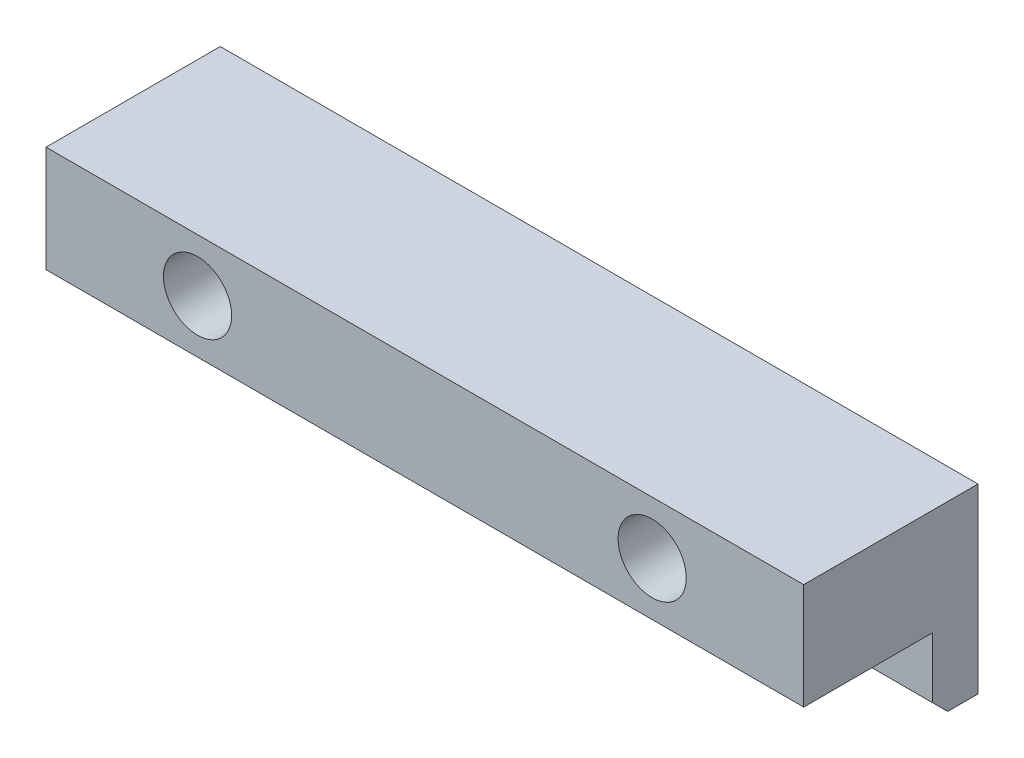
from build123d import *

# Parameters (mm, degrees)
SKETCH1_W           = 50
SKETCH1_H           = 12
BOSS_EXTRUDE1_DEPTH = 5
SKETCH2_R           = 2.25
CUT_EXTRUDE1_DEPTH  = 52.662365412
SKETCH3_W           = 2
SKETCH3_H           = 5
CUT_EXTRUDE2_DEPTH  = 52.662365412
CHAMFER1_SIZE       = 1
MOVE_FACE1_BY       = 6.5


with BuildPart() as part:
    # Sketch1 → Boss-Extrude1 (new body)
    with BuildSketch(Plane.XY):
        with Locations((25, 6)):
            Rectangle(SKETCH1_W, SKETCH1_H)
    extrude(amount=BOSS_EXTRUDE1_DEPTH)

    # Sketch2 → Cut-Extrude1 (cut, through all)
    with BuildSketch(Plane.XY.offset(5)):
        with Locations((10, 8.5)):
            Circle(SKETCH2_R)
        with Locations((40, 8.5)):
            Circle(SKETCH2_R)
    extrude(amount=-CUT_EXTRUDE1_DEPTH, mode=Mode.SUBTRACT)

    # Sketch3 → Cut-Extrude2 (cut, through all)
    with BuildSketch(Plane(origin=(50, 0, 0), x_dir=(0, 0, -1), z_dir=(1, 0, 0))):
        with Locations((-4, 2.5)):
            Rectangle(SKETCH3_W, SKETCH3_H)
    extrude(amount=-CUT_EXTRUDE2_DEPTH, mode=Mode.SUBTRACT)

    # Chamfer1
    chamfer1_edges = [part.edges().sort_by_distance(p)[0] for p in [
        (25, 0, 3),
    ]]
    chamfer(chamfer1_edges, length=CHAMFER1_SIZE)

    # Move Face1: a face moved outward by 6.5
    extrude(part.faces().sort_by_distance((25, 8.5, 5))[0], amount=MOVE_FACE1_BY, dir=(0, 0, 1))


solid = part.part
